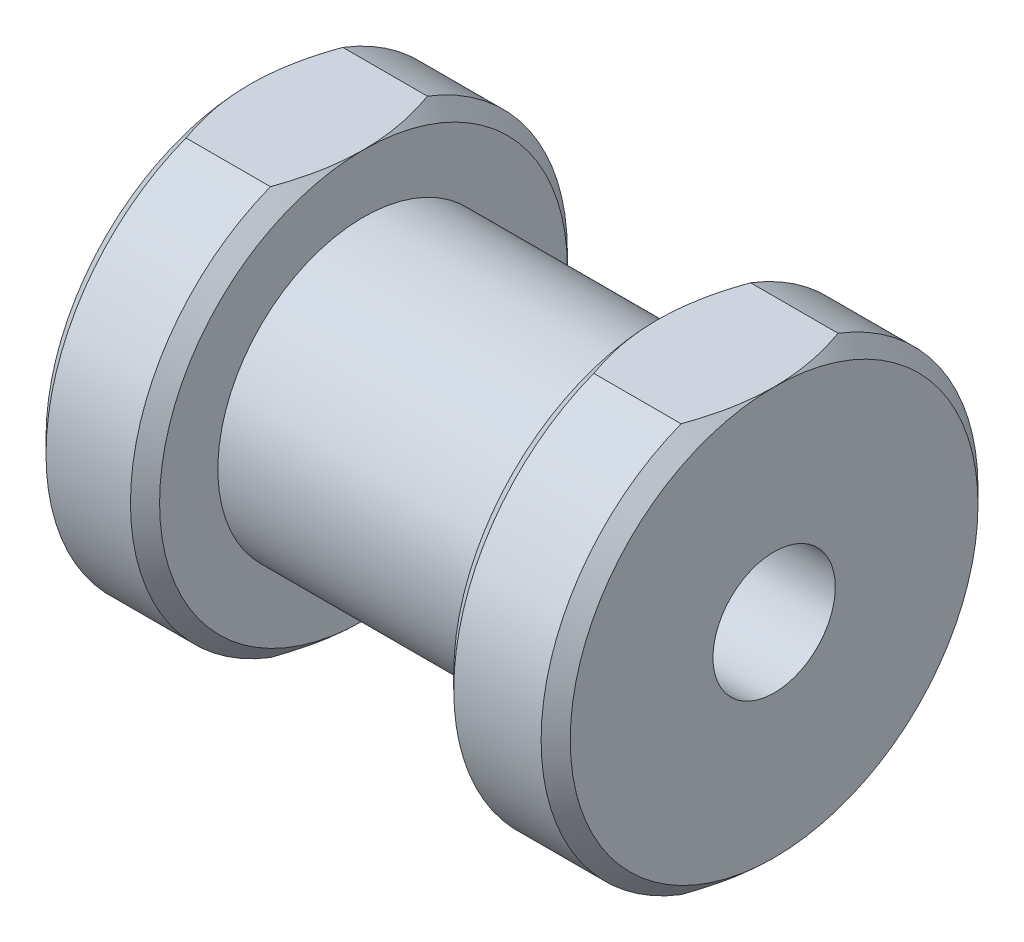
from build123d import *

# Parameters (mm, degrees)
SKETCH_1_R           = 7.5
EXTRUDE_1_DEPTH      = 18
HOLE_WIZARD_M5_1_D   = 4.2
CUT_EXTRUDE_START    = -4
SKETCH_5_OUTSIDE_W   = 22.564
SKETCH_5_OUTSIDE_H   = 22.564
SKETCH_5_OUTSIDE_R   = 5
CUT_EXTRUDE_1_DEPTH  = 10.1
CHAMFER_1_SIZE       = 0.5
SKETCH_6_OUTSIDE_W   = 22.564
SKETCH_6_OUTSIDE_H   = 22.564
SKETCH_6_OUTSIDE_W_2 = 30.328855636
SKETCH_6_OUTSIDE_H_2 = 14
CUT_EXTRUDE_2_DEPTH  = 21.892582416


with BuildPart() as part:
    # 草图1 → 凸台-拉伸1 (new body)
    with BuildSketch(Plane(origin=(0, 0, 0), x_dir=(0, 0, -1), z_dir=(1, 0, 0))):
        Circle(SKETCH_1_R)
    extrude(amount=EXTRUDE_1_DEPTH)

    # M5 螺纹孔1 (through all)
    with Locations(Plane(origin=(18, 0, 0), x_dir=(0, 0, -1), z_dir=(1, 0, 0))):
        with Locations((0, 0)):
            Hole(HOLE_WIZARD_M5_1_D / 2)

    # 草图5 outside → 切除-拉伸1 (cut)
    with BuildSketch(Plane(origin=(18, 0, 0), x_dir=(0, 0, -1), z_dir=(1, 0, 0)).offset(CUT_EXTRUDE_START)):
        Rectangle(SKETCH_5_OUTSIDE_W, SKETCH_5_OUTSIDE_H)
        Circle(SKETCH_5_OUTSIDE_R, mode=Mode.SUBTRACT)
    extrude(amount=-CUT_EXTRUDE_1_DEPTH, mode=Mode.SUBTRACT)

    # 倒角1
    chamfer_1_edges = [part.edges().sort_by_distance(p)[0] for p in [
        (14, 0, 7.5),
        (3.9, 0, 7.5),
        (0, 0, 7.5),
        (18, 0, 7.5),
    ]]
    chamfer(chamfer_1_edges, length=CHAMFER_1_SIZE)

    # 草图6 outside → 切除-拉伸2 (cut, through all)
    with BuildSketch(Plane(origin=(18, 0, 0), x_dir=(0, 0, -1), z_dir=(1, 0, 0))):
        Rectangle(SKETCH_6_OUTSIDE_W, SKETCH_6_OUTSIDE_H)
        Rectangle(SKETCH_6_OUTSIDE_W_2, SKETCH_6_OUTSIDE_H_2, mode=Mode.SUBTRACT)
    extrude(amount=-CUT_EXTRUDE_2_DEPTH, mode=Mode.SUBTRACT)


solid = part.part
